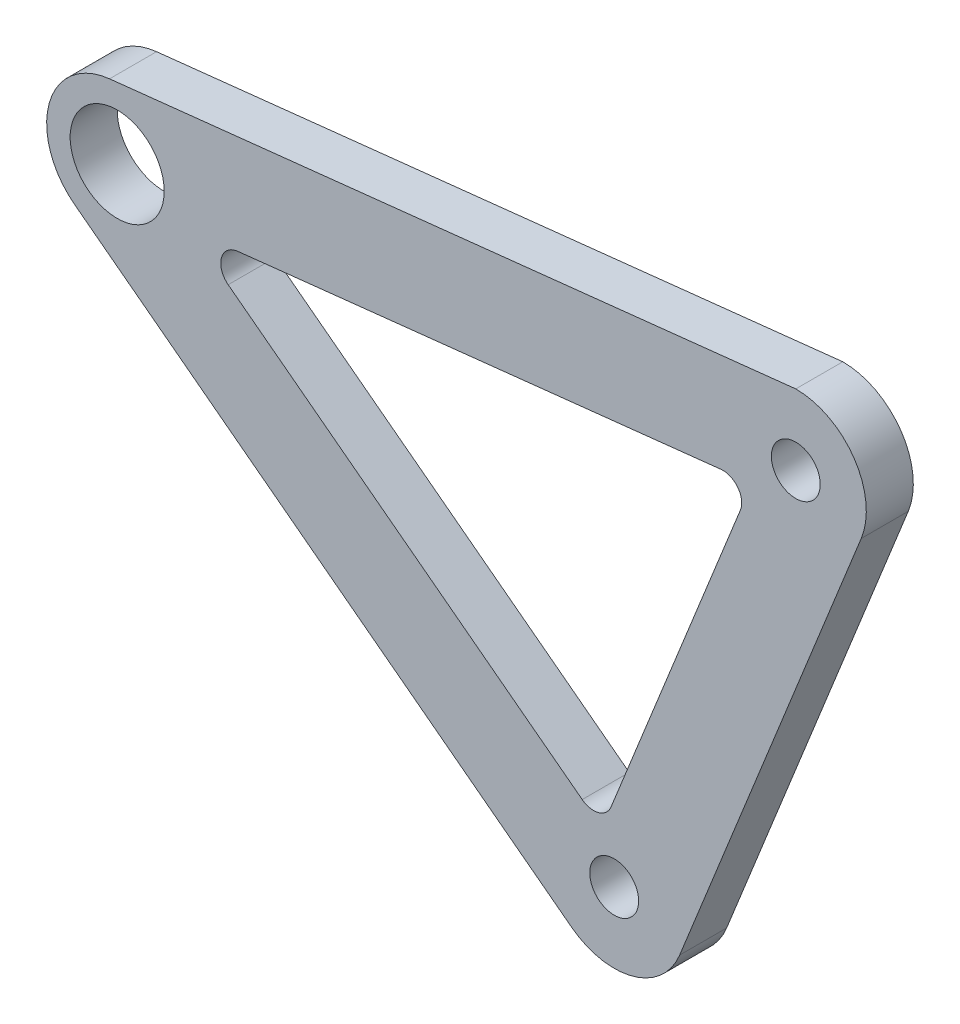
from build123d import *

# Parameters (mm, degrees)
SKETCH1_R           = 2.6
SKETCH1_R_2         = 5
BOSS_EXTRUDE1_DEPTH = 5


with BuildPart() as part:
    # Sketch1 → Boss-Extrude1 (new body)
    with BuildSketch(Plane.XY):
        with BuildLine():
            Line((-72.991378041, -0.434123458), (0, 7.5))
            ThreePointArc((0, 7.5), (6.214243254, 4.199188109), (6.958607035, -2.79781846))
            Line((6.958607035, -2.79781846), (-12.355075838, -50.833933534))
            ThreePointArc((-12.355075838, -50.833933534), (-17.316674975, -55.265358427), (-23.849430907, -54.009136903))
            Line((-23.849430907, -54.009136903), (-76.716654152, -13.863225709))
            ThreePointArc((-76.716654152, -13.863225709), (-79.407988086, -5.885388122), (-72.991378041, -0.434123458))
        make_face()
        Circle(SKETCH1_R, mode=Mode.SUBTRACT)
        with Locations((-19.313682873, -48.036115074)):
            Circle(SKETCH1_R, mode=Mode.SUBTRACT)
        with Locations((-72.180906117, -7.89020388)):
            Circle(SKETCH1_R_2, mode=Mode.SUBTRACT)
        with BuildLine():
            Line((-7.969347023, -3.889011646), (-59.380826719, -9.508878151))
            ThreePointArc((-59.380826719, -9.508878151), (-61.090881727, -10.963000514), (-60.373031081, -13.089840994))
            Line((-60.373031081, -13.089840994), (-22.717890398, -41.684116257))
            ThreePointArc((-22.717890398, -41.684116257), (-20.97582215, -42.019108663), (-19.652729047, -40.837395359))
            Line((-19.652729047, -40.837395359), (-5.896390033, -6.623253591))
            ThreePointArc((-5.896390033, -6.623253591), (-6.1582725, -4.668875059), (-7.969347023, -3.889011646))
        make_face(mode=Mode.SUBTRACT)
    extrude(amount=BOSS_EXTRUDE1_DEPTH)


solid = part.part
